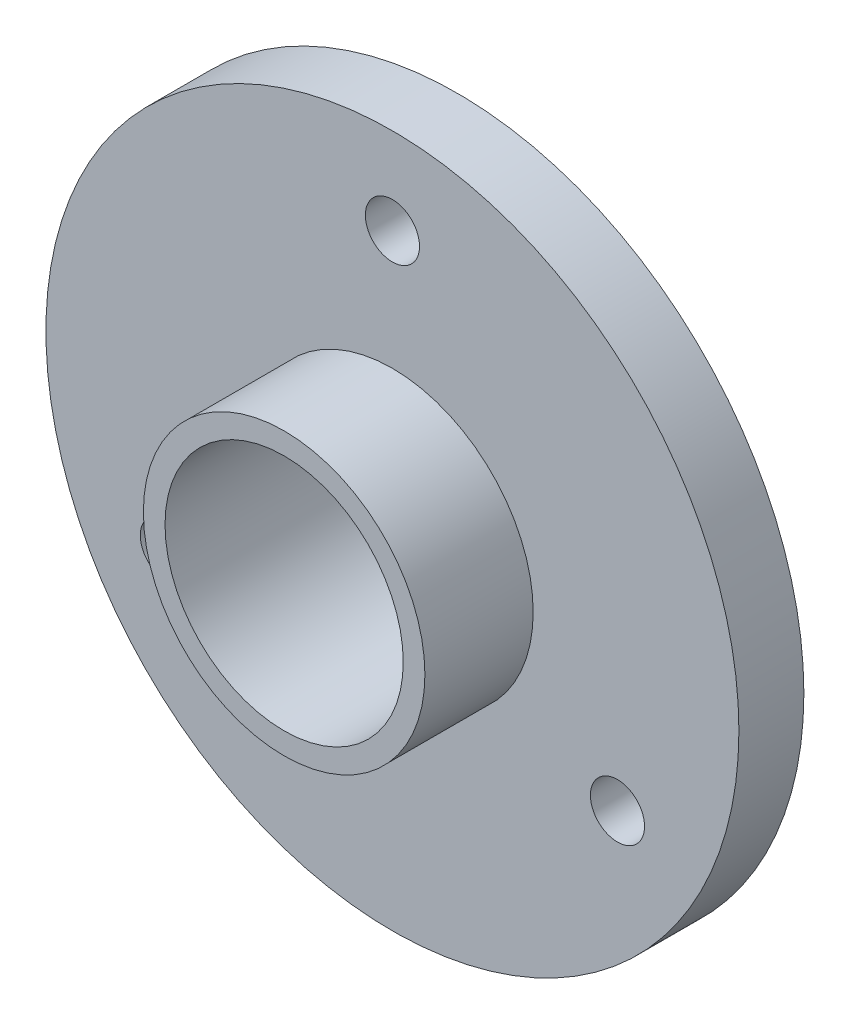
SolidWorks part; units mm, degrees
ref_plane "Front Plane" through (0, 0, 0) normal (0, 0, 1) x (1, 0, 0)
ref_plane "Top Plane" through (0, 0, 0) normal (0, 1, 0) x (1, 0, 0)
ref_plane "Right Plane" through (0, 0, 0) normal (1, 0, 0) x (0, 0, -1)
sketch "Sketch1" plane through (0, 0, 0) normal (0, 0, 1) x (1, 0, 0)
  circle A0 centre (0, 0) radius 16
  dimension "D1" = 32
extrude "Boss-Extrude1" add sketch "Sketch1" along normal blind 3
sketch "Sketch2" plane through (0, 0, 3) normal (0, 0, 1) x (1, 0, 0)
  circle A0 centre (0, 0) radius 6.5
  dimension "D1" = 13
extrude "Boss-Extrude2" add sketch "Sketch2" along normal blind 5
sketch "Sketch3" plane through (0, 0, 0) normal (0, 0, -1) x (-1, 0, 0)
  circle A0 centre (0, 0) radius 5.5
  dimension "D1" = 11
extrude "Cut-Extrude1" cut sketch "Sketch3" against normal blind 22
sketch "Sketch4" plane through (0, 0, 0) normal (0, 0, -1) x (-1, 0, 0)
  circle A0 centre (0, 12) radius 1
  circle A1 centre (10.3923, -6) radius 1
  circle A2 centre (-10.3923, -6) radius 1
  point P10 (0, 0)
  dimension "D2" = 2
  dimension "D1" = 12
  dimension "D3" = 3
extrude "Cut-Extrude2" cut sketch "Sketch4" against normal blind 10
hole_wizard "M3 Tapped Hole1" positions "Sketch6" profile "Sketch5" tap size "M3" standard "GB" end condition up to next
sketch "Sketch6" plane through (0, 0, 0) normal (0, 0, -1) x (-1, 0, 0)
  point P0 (0, 12)
  point P3 (10.3923, -6)
  point P6 (-10.3923, -6)
sketch "Sketch5" plane through (0, 12, 0) normal (1, 0, 0) x (0, 1, 0)
  line L0 (0, 0) -> (0, 8)
  line L1 (0, 8) -> (1.25, 8)
  line L2 (1.25, 8) -> (1.25, 0)
  line L5 (1.25, 0) -> (0, 0)
  line L11 (0, -6.35) -> (0, 107.95) construction
  dimension "通孔螺纹孔钻头直径" = 2.5
  dimension "通孔螺纹孔钻头深度" = 8
cosmetic thread "CosmeticThread1" parameters "D2"=3
cosmetic thread "CosmeticThread2" parameters "D2"=3
cosmetic thread "CosmeticThread3" parameters "D2"=3
